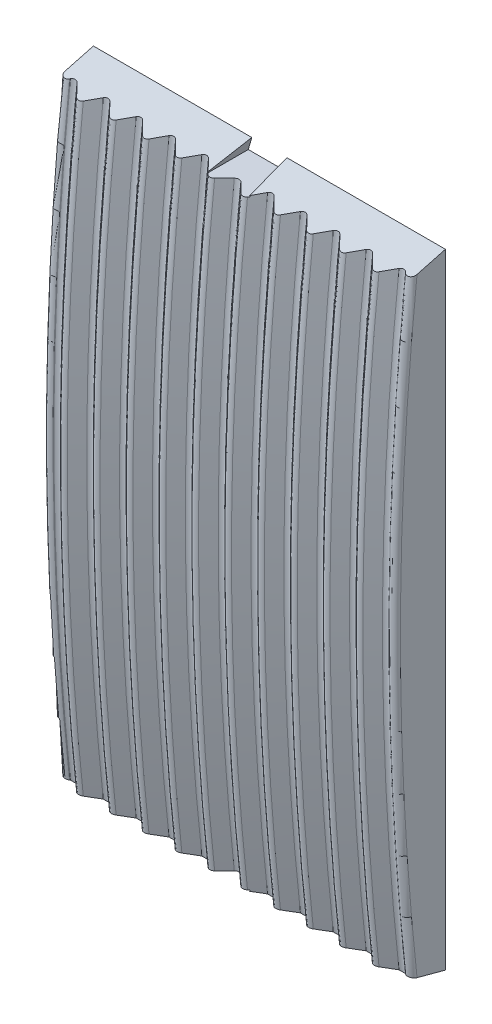
SolidWorks part; units mm, degrees
material "ZGMn13-2"
ref_plane "Front Plane" through (0, 0, 0) normal (0, 0, 1) x (1, 0, 0)
ref_plane "Top Plane" through (0, 0, 0) normal (0, 1, 0) x (1, 0, 0)
ref_plane "Right Plane" through (0, 0, 0) normal (1, 0, 0) x (0, 0, -1)
sketch "Sketch2" plane through (0, 0, 0) normal (1, 0, 0) x (0, 0, -1)
  line L0 (0, -142.9093) -> (0, 142.9093) construction
  line L1 (130, 0) -> (-130, 0) construction
  line L2 (130, -665) -> (130, 665)
  line L3 (130, 665) -> (34.158, 639.3192)
  line L4 (130, -665) -> (34.158, -639.3192)
  arc A0 (34.158, 639.3192) -> (34.158, -639.3192) centre (6000, 0) ccw
  point P4 (0, 0)
  point P8 (0, 0)
  point P11 (130, 0)
  dimension "D3" = 6000
  dimension "D1" = 1330
  dimension "D2" = 75
  dimension "D4" = 130
extrude "Boss-Extrude1" add sketch "Sketch2" along normal mid plane 750
sketch "Sketch3" plane through (0, 0, -130) normal (0, 0, -1) x (-1, 0, 0)
  line L0 (0, -797.3156) -> (0, 797.3156) construction
  line L1 (-37.5, 665) -> (-45, 639)
  line L2 (-375, 665) -> (375, 665) construction
  line L3 (-45, 639) -> (45, 639)
  line L4 (45, 639) -> (37.5, 665)
  line L5 (37.5, 665) -> (-37.5, 665)
  point P4 (0, 0)
  dimension "D1" = 75
  dimension "D2" = 90
  dimension "D3" = 26
extrude "Cut-Extrude1" cut sketch "Sketch3" against normal blind 750
mirror "Mirror1" about plane through (0, 0, 0) normal (0, 1, 0) of "Cut-Extrude1"
sketch "Sketch4" plane through (0, 0, 0) normal (1, 0, 0) x (0, 0, -1)
  arc A0 (34.158, 639.3192) -> (34.158, -639.3192) centre (6000, 0) ccw construction
  arc A1 (36.966, 665) -> (36.966, -665) centre (6000, 0) ccw
sketch "Sketch5" plane through (0, 0, 0) normal (0, 1, 0) x (1, 0, 0)
  line L0 (0, 0) -> (0, 145.3257) construction
  line L1 (0, 35) -> (-35, 0)
  line L3 (-35, 0) -> (35, 0)
  line L4 (35, 0) -> (0, 35)
  dimension "D1" = 70
  dimension "D2" = 35
sweep "Cut-Sweep1" cut profiles "Sketch5" path "Sketch4"
pattern_linear "LPattern1" count 6 spacing 70 along (-1, 0, 0) of "Cut-Sweep1"
pattern_linear "LPattern2" count 6 spacing 70 along (1, 0, 0) of "Cut-Sweep1"
fillet "Fillet1" radius 10 23 edges at (-350, 0, -35) (-375, 0, -10) (140, 0, -35) (210, 0, -35) (280, 0, -35) (350, 0, -35) (375, 0, -10) (315, 0, 0) (245, 0, 0) (175, 0, 0) (70, 0, -35) (0, 0, -35) (105, 0, 0) (35, 0, 0) (-35, 0, 0) (-70, 0, -35) (-105, 0, 0) (-140, 0, -35) (-175, 0, 0) (-210, 0, -35) (-245, 0, 0) (-280, 0, -35) (-315, 0, 0)
sketch "Sketch6" plane through (0, 0, -130) normal (0, 0, -1) x (-1, 0, 0)
  line L0 (0, -723.8907) -> (0, 723.8907) construction
  line L1 (449.5012, 0) -> (-449.5012, 0) construction
  line L3 (335, -125) -> (20, -125)
  line L4 (335, -125) -> (335, 125)
  line L5 (335, 125) -> (20, 125)
  line L6 (20, -125) -> (20, 125)
  line L7 (335, -125) -> (20, 125) construction
  line L8 (335, 125) -> (20, -125) construction
  line L9 (-20, -125) -> (-335, -125)
  line L10 (-20, -125) -> (-20, 125)
  line L11 (-20, 125) -> (-335, 125)
  line L12 (-335, -125) -> (-335, 125)
  line L13 (-20, -125) -> (-335, 125) construction
  line L14 (-20, 125) -> (-335, -125) construction
  point P0 (177.5, 0)
  point P4 (0, 0)
  point P10 (-177.5, 0)
  point P18 (0, 0)
  dimension "D1" = 250
  dimension "D2" = 315
  dimension "D3" = 40
  dimension "D4" = 315
extrude "Cut-Extrude2" cut sketch "Sketch6" against normal blind 60
sketch "Sketch7" plane through (0, 0, 0) normal (1, 0, 0) x (0, 0, -1)
  line L0 (130, 625) -> (130, 455)
  line L1 (130, -665) -> (130, 665) construction
  line L2 (130, 455) -> (87.4815, 455)
  line L3 (130, 625) -> (103.0283, 625)
  line L4 (130, 415) -> (130, 165)
  line L5 (130, 165) -> (72.296, 165)
  line L6 (130, 415) -> (84.5393, 415)
  line L7 (0, 0) -> (286.5873, 0) construction
  arc A0 (87.4815, 455) -> (103.0283, 625) centre (6000, 0) cw
  arc A1 (69.5258, 648.796) -> (69.5258, -648.796) centre (6000, 0) ccw construction
  arc A2 (72.296, 165) -> (84.5393, 415) centre (6000, 0) cw
  dimension "D1" = 5930
  dimension "D4" = 5930
  dimension "D2" = 455
  dimension "D3" = 170
  dimension "D5" = 40
  dimension "D6" = 250
extrude "Cut-Extrude3" cut sketch "Sketch7" against normal mid plane 670
sketch "Sketch8" plane through (0, 0, -130) normal (0, 0, -1) x (-1, 0, 0)
  line L0 (0, -728.38) -> (0, 728.38) construction
  line L1 (475.199, 0) -> (-475.199, 0) construction
  line L2 (335, 625) -> (-335, 625) construction
  line L3 (-20, 625) -> (20, 625)
  line L4 (-20, 625) -> (-20, 455)
  line L5 (-20, 455) -> (20, 455)
  line L6 (20, 625) -> (20, 455)
  line L7 (335, 455) -> (-335, 455) construction
  line L8 (335, 415) -> (-335, 415) construction
  line L9 (-135, 415) -> (-100, 415)
  line L10 (-135, 415) -> (-135, 165)
  line L11 (-135, 165) -> (-100, 165)
  line L12 (-100, 415) -> (-100, 165)
  line L13 (335, 165) -> (-335, 165) construction
  line L15 (100, 415) -> (135, 415)
  line L16 (100, 415) -> (100, 165)
  line L17 (100, 165) -> (135, 165)
  line L18 (135, 415) -> (135, 165)
  point P4 (0, 0)
  point P8 (0, 0)
  dimension "D1" = 40
  dimension "D2" = 35
  dimension "D3" = 200
  dimension "D4" = 35
extrude "Boss-Extrude2" add sketch "Sketch8" against normal up to surface (26.9717 mm away)
mirror "Mirror3" about plane through (0, 0, 0) normal (0, 1, 0) of "Cut-Extrude3", "Boss-Extrude2"
